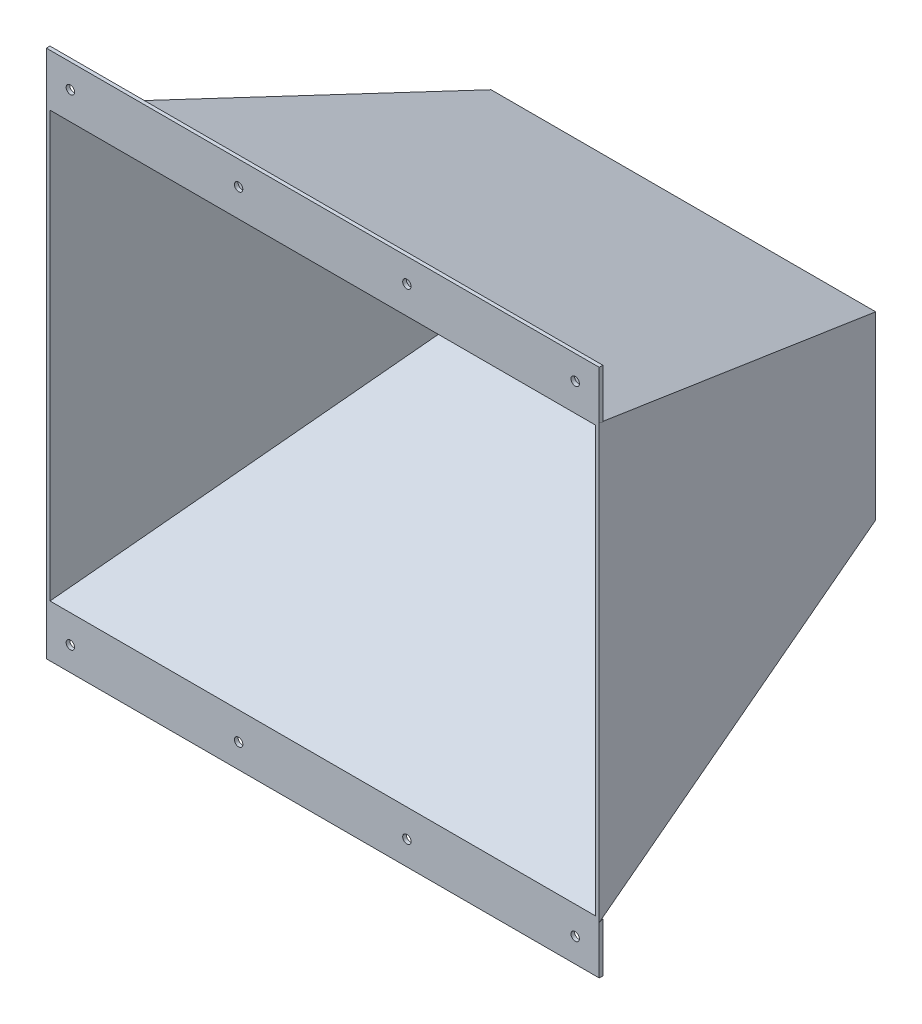
SolidWorks part; units mm, degrees
ref_plane "Front Plane" through (0, 0, 0) normal (0, 0, 1) x (1, 0, 0)
ref_plane "Top Plane" through (0, 0, 0) normal (0, 1, 0) x (1, 0, 0)
ref_plane "Right Plane" through (0, 0, 0) normal (1, 0, 0) x (0, 0, -1)
sketch "Sketch1" plane through (0, 0, 0) normal (0, 0, 1) x (1, 0, 0)
  line L1 (-230, 180) -> (230, 180)
  line L2 (-230, 180) -> (-230, -180)
  line L3 (-230, -180) -> (230, -180)
  line L4 (230, 180) -> (230, -180)
  line L5 (-230, 180) -> (230, -180) construction
  line L6 (-230, -180) -> (230, 180) construction
  point P0 (0, 0)
  dimension "D1" = 360
  dimension "D2" = 460
extrude "Boss-Extrude1" add sketch "Sketch1" against normal blind 300
sketch "Sketch3" plane through (230, 0, 0) normal (1, 0, 0) x (0, 0, -1)
  line L0 (0, 180) -> (300, 75)
  line L1 (300, -180) -> (300, 180) construction
  line L2 (300, 75) -> (300, 180)
  line L3 (300, 180) -> (0, 180)
  line L4 (0, 0) -> (300, 0) construction
  line L5 (300, -180) -> (0, -180)
  line L6 (300, -75) -> (300, -180)
  line L7 (0, -180) -> (300, -75)
  dimension "D1" = 150
extrude "Cut-Extrude1" cut sketch "Sketch3" against normal through all
sketch "Sketch6" plane through (0, 0, 0) normal (0, 1, 0) x (1, 0, 0)
  line L0 (-230, 0) -> (-160, 300)
  line L1 (-230, 300) -> (230, 300) construction
  line L2 (-160, 300) -> (-230, 300)
  line L3 (-230, 300) -> (-230, 0)
  line L4 (0, 0) -> (0, 202.4784) construction
  line L5 (230, 300) -> (230, 0)
  line L6 (160, 300) -> (230, 300)
  line L7 (230, 0) -> (160, 300)
  dimension "D1" = 320
extrude "Cut-Extrude3" cut sketch "Sketch6" against normal mid plane 604
shell "Shell1" thickness 3
sketch "Sketch7" plane through (0, 0, -297) normal (0, 0, 1) x (1, 0, 0)
  line L4 (157.6194, 72.8716) -> (-157.6194, 72.8716)
  line L5 (-157.6194, 72.8716) -> (-157.6194, -72.8716)
  line L6 (-157.6194, -72.8716) -> (157.6194, -72.8716)
  line L7 (157.6194, -72.8716) -> (157.6194, 72.8716)
  line L8 (157.6194, 72.8716) -> (-157.6194, 72.8716)
  line L9 (-157.6194, 72.8716) -> (-157.6194, -72.8716)
  line L10 (-157.6194, -72.8716) -> (157.6194, -72.8716)
  line L11 (157.6194, -72.8716) -> (157.6194, 72.8716)
  dimension "D1" = 0
extrude "Cut-Extrude4" cut sketch "Sketch7" against normal through all
sketch "Sketch8" plane through (0, 0, 0) normal (0, 0, 1) x (1, 0, 0)
  line L1 (-230, -180) -> (230, -180)
  line L2 (-230, -180) -> (-230, -220)
  line L3 (-230, -220) -> (230, -220)
  line L4 (230, -180) -> (230, -220)
  dimension "D1" = 40
extrude "Boss-Extrude2" add sketch "Sketch8" against normal blind 3
sketch "Sketch9" plane through (0, -180, 0) normal (0, 1, 0) x (1, 0, 0)
  line L4 (-230, 0) -> (230, 0)
  line L5 (230, 0) -> (230, 3)
  line L6 (230, 3) -> (-230, 3)
  line L7 (-230, 3) -> (-230, 0)
  line L8 (-230, 0) -> (230, 0)
  line L9 (230, 0) -> (230, 3)
  line L10 (230, 3) -> (-230, 3)
  line L11 (-230, 3) -> (-230, 0)
  dimension "D1" = 0
extrude "Boss-Extrude3" add sketch "Sketch9" along normal up to surface (1.05 mm away)
sketch "Sketch10" plane through (0, 0, 0) normal (0, 0, 1) x (1, 0, 0)
  line L1 (-230, 180) -> (230, 180)
  line L2 (-230, 180) -> (-230, 220)
  line L3 (-230, 220) -> (230, 220)
  line L4 (230, 180) -> (230, 220)
  dimension "D1" = 40
extrude "Boss-Extrude4" add sketch "Sketch10" against normal blind 3 separate body
sketch "Sketch11" plane through (0, 180, 0) normal (0, -1, 0) x (1, 0, 0)
  line L4 (230, 0) -> (-230, 0)
  line L5 (-230, 0) -> (-230, -3)
  line L6 (-230, -3) -> (230, -3)
  line L7 (230, -3) -> (230, 0)
  line L8 (230, 0) -> (-230, 0)
  line L9 (-230, 0) -> (-230, -3)
  line L10 (-230, -3) -> (230, -3)
  line L11 (230, -3) -> (230, 0)
  dimension "D1" = 0
extrude "Boss-Extrude5" add sketch "Sketch11" along normal up to surface (1.05 mm away)
hole_wizard "Ø7.0 (7) Diameter Hole1" positions "Sketch14" profile "Sketch13" hole size "Ø7.0" standard "Gb" end condition through all
sketch "Sketch14" plane through (0, 0, 0) normal (0, 0, 1) x (1, 0, 0)
  line L0 (-230, 220) -> (-230, 180) construction
  line L2 (230, 220) -> (-230, 220) construction
  point P0 (-210, 200)
  dimension "D1" = 20
  dimension "D2" = 20
sketch "Sketch13" plane through (-210, 200, 0) normal (1, 0, 0) x (0, -1, 0)
  line L0 (0, 0) -> (0, 300)
  line L1 (0, 300) -> (3.5, 300)
  line L2 (3.5, 300) -> (3.5, 0)
  line L5 (3.5, 0) -> (0, 0)
  line L11 (0, -6.35) -> (0, 107.95) construction
  dimension "通孔孔直径" = 7
  dimension "通孔孔深度" = 300
pattern_linear "LPattern1" count 4 spacing 140 along (1, 0, 0) of "Ø7.0 (7) Diameter Hole1"
mirror "Mirror5" about plane through (0, 0, 0) normal (0, 1, 0) of "LPattern1", "Ø7.0 (7) Diameter Hole1"
